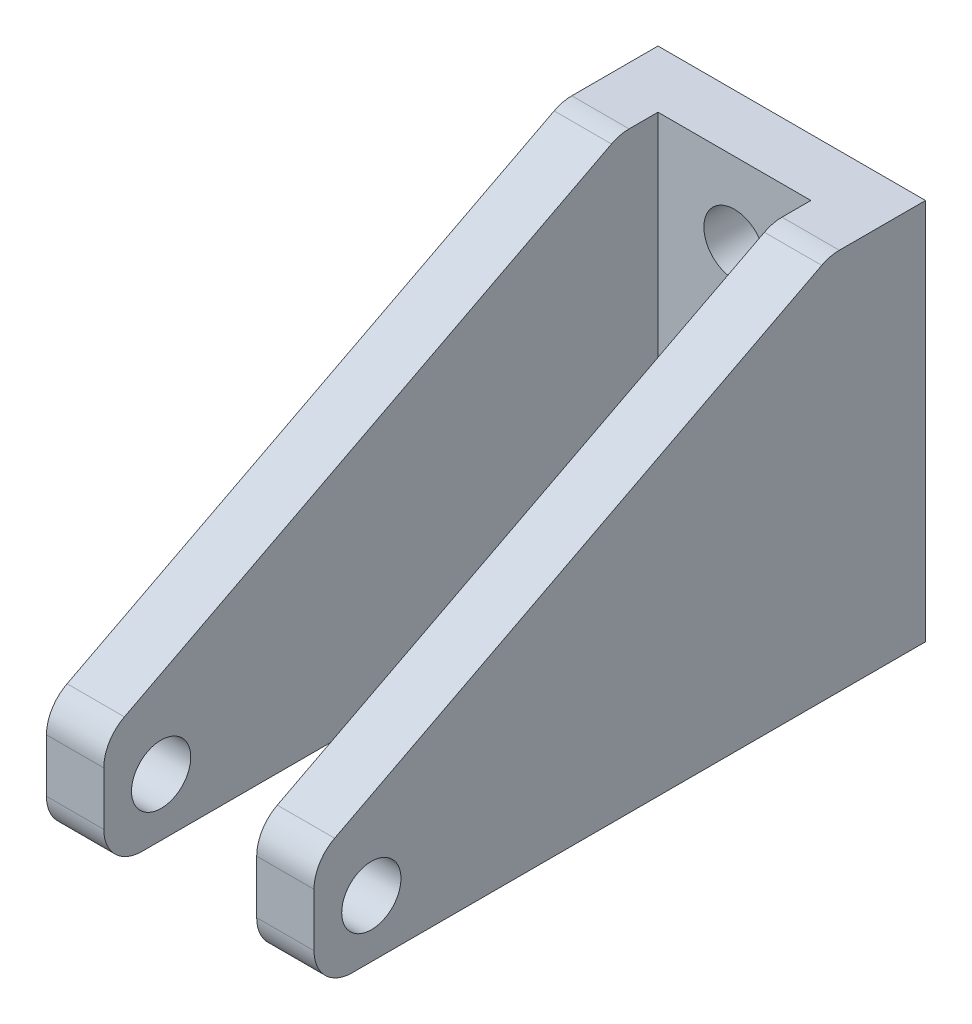
from build123d import *

# Parameters (mm, degrees)
SKETCH_1_W          = 14
SKETCH_1_H          = 32
EXTRUDE_1_DEPTH     = 20
CUT_EXTRUDE_1_DEPTH = 20
SKETCH_3_W          = 8
SKETCH_3_H          = 29
CUT_EXTRUDE_2_DEPTH = 20
FILLET_2_R          = 2
SKETCH_4_R          = 1.55
CUT_EXTRUDE_3_DEPTH = 20
SKETCH_5_R          = 1.6
CUT_EXTRUDE_4_DEPTH = 20


with BuildPart() as part:
    # 草图1 → 凸台-拉伸1 (new body)
    with BuildSketch(Plane(origin=(0, 0, 0), x_dir=(1, 0, 0), z_dir=(0, 1, 0))):
        Rectangle(SKETCH_1_W, SKETCH_1_H)
    extrude(amount=EXTRUDE_1_DEPTH)

    # 草图2 → 切除-拉伸1 (cut)
    with BuildSketch(Plane(origin=(7, 0, 0), x_dir=(0, 0, -1), z_dir=(1, 0, 0))):
        Polygon((-16, 6), (11, 20), (-16, 20), align=None)
    extrude(amount=-CUT_EXTRUDE_1_DEPTH, mode=Mode.SUBTRACT)

    # 草图3 → 切除-拉伸2 (cut)
    with BuildSketch(Plane.XZ):
        with Locations((0, 1.5)):
            Rectangle(SKETCH_3_W, SKETCH_3_H)
    extrude(amount=-CUT_EXTRUDE_2_DEPTH, mode=Mode.SUBTRACT)

    # 圆角2
    fillet_2_edges = [part.edges().sort_by_distance(p)[0] for p in [
        (-5.5, 20, -11),
        (-5.5, 6, 16),
        (5.5, 6, 16),
        (5.5, 20, -11),
        (5.5, 0, 16),
        (-5.5, 0, 16),
    ]]
    fillet(fillet_2_edges, radius=FILLET_2_R)

    # 草图4 → 切除-拉伸3 (cut)
    with BuildSketch(Plane.ZY.offset(7)):
        with Locations((13, 3)):
            Circle(SKETCH_4_R)
    extrude(amount=-CUT_EXTRUDE_3_DEPTH, mode=Mode.SUBTRACT)

    # 草图5 → 切除-拉伸4 (cut)
    with BuildSketch(Plane.XY.offset(-13)):
        with Locations((0, 16)):
            Circle(SKETCH_5_R)
        with Locations((0, 6)):
            Circle(SKETCH_5_R)
    extrude(amount=-CUT_EXTRUDE_4_DEPTH, mode=Mode.SUBTRACT)


solid = part.part
